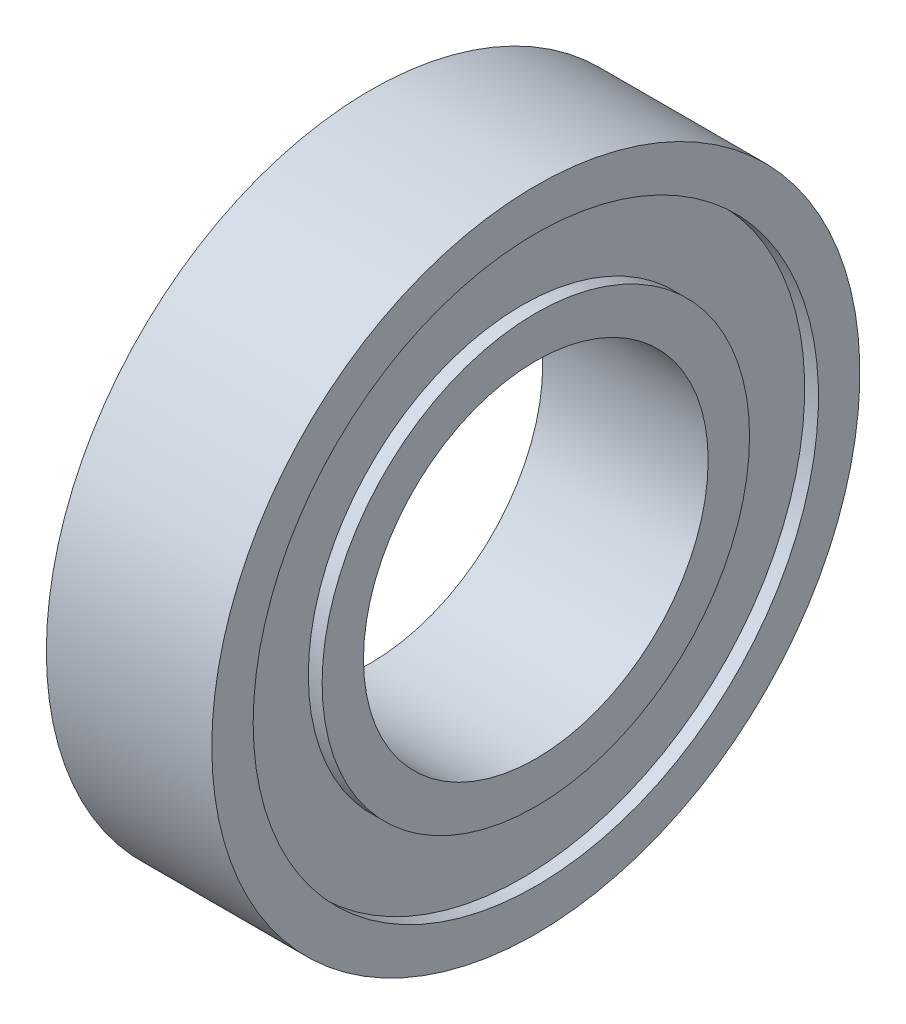
from build123d import *


with BuildPart() as part:
    # Sketch1 → Revolve1 (revolve)
    with BuildSketch(Plane.XY, mode=Mode.PRIVATE) as revolve1_sk:
        Polygon((13.120246846, 20.5), (13.120246846, 23.5), (25.120246846, 23.5), (25.120246846, 20.5), (24.120246846, 20.5), (24.120246846, 15.5), (25.120246846, 15.5), (25.120246846, 12.5), (13.120246846, 12.5), (13.120246846, 15.5), (14.120246846, 15.5), (14.120246846, 20.5), align=None)
    revolve(revolve1_sk.sketch.rotate(Axis((0, 0, 0), (1, 0, 0)), 90), axis=Axis((0, 0, 0), (1, 0, 0)))


solid = part.part
